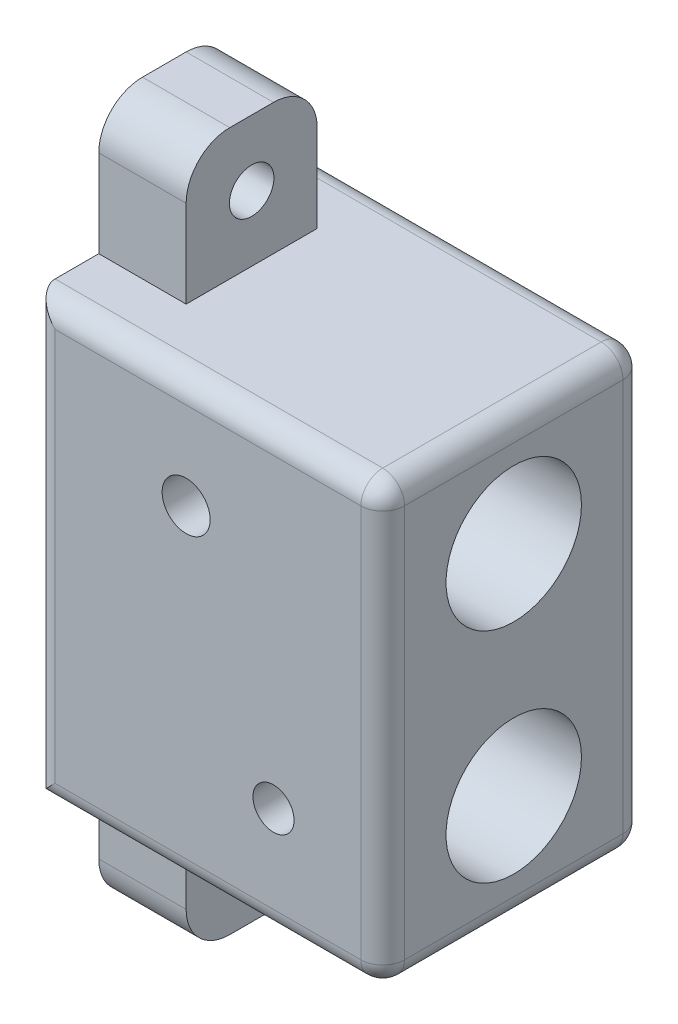
SolidWorks part; units mm, degrees
ref_plane "Front Plane" through (0, 0, 0) normal (0, 0, 1) x (1, 0, 0)
ref_plane "Top Plane" through (0, 0, 0) normal (0, 1, 0) x (1, 0, 0)
ref_plane "Right Plane" through (0, 0, 0) normal (1, 0, 0) x (0, 0, -1)
sketch "Sketch1" plane through (0, 0, 0) normal (0, 1, 0) x (1, 0, 0)
  line L0 (0, 20) -> (20, 20)
  line L2 (0, 0) -> (0, 20)
  line L4 (20, 0) -> (20, 20)
  line L5 (20, 0) -> (80, 0)
  line L6 (0, 0) -> (0, -60)
  line L7 (0, -60) -> (80, -60)
  line L8 (80, 0) -> (80, -60)
  dimension "D1" = 20
  dimension "D2" = 80
  dimension "D3" = 20
  dimension "D4" = 60
extrude "Boss-Extrude1" add sketch "Sketch1" along normal blind 100
sketch "Sketch2" plane through (80, 0, 0) normal (1, 0, 0) x (0, 0, -1)
  line L0 (0, 100) -> (0, 0) construction
  line L1 (0, 100) -> (0, 0) construction
  line L2 (-60, 0) -> (0, 0) construction
  line L3 (-60, 100) -> (0, 100) construction
  circle A0 centre (-30, 75) radius 15.5
  circle A1 centre (-30, 25) radius 15.5
  dimension "D1" = 31
  dimension "D2" = 31
  dimension "D4" = 30
  dimension "D5" = 25
  dimension "D6" = 25
  dimension "D3" = 30
extrude "Cut-Extrude1" cut sketch "Sketch2" against normal blind 70
sketch "Sketch3" plane through (20, 0, 0) normal (1, 0, 0) x (0, 0, -1)
  line L0 (20, 100) -> (20, 0) construction
  line L1 (0, 0) -> (20, 0) construction
  circle A0 centre (10, 87.5) radius 5.1
  circle A1 centre (10, 12.5) radius 5.1
  circle A2 centre (10, 50) radius 5.1
  dimension "D1" = 10
  dimension "D2" = 10
  dimension "D3" = 10.2
  dimension "D4" = 10.2
  dimension "D5" = 75
  dimension "D6" = 12.5
  dimension "D7" = 10
  dimension "D8" = 37.5
  dimension "D9" = 10.2
extrude "Cut-Extrude2" cut sketch "Sketch3" against normal blind 70
sketch "Sketch4" plane through (0, 0, 0) normal (0, 0, -1) x (-1, 0, 0)
  line L0 (-80, 100) -> (-80, 0) construction
  line L1 (-80, 0) -> (-20, 0) construction
  line L2 (-80, 100) -> (-20, 100) construction
  circle A0 centre (-35, 75) radius 5.5
  circle A1 centre (-55, 25) radius 4.7053
  dimension "D1" = 11
  dimension "D2" = 45
  dimension "D3" = 25
  dimension "D4" = 25
  dimension "D5" = 25
extrude "Cut-Extrude3" cut sketch "Sketch4" against normal blind 70
sketch "Sketch5" plane through (0, 0, 0) normal (-1, 0, 0) x (0, 0, 1)
  line L0 (60, 100) -> (60, 0) construction
  line L1 (35, 130) -> (25, 130)
  line L2 (45, 120) -> (45, -20)
  line L3 (35, -30) -> (25, -30)
  line L4 (15, 120) -> (15, -20)
  line L5 (-20, 0) -> (60, 0) construction
  line L6 (-20, 100) -> (60, 100) construction
  circle A0 centre (30, -15) radius 5.1
  circle A1 centre (30, 115) radius 5.1
  arc A2 (25, 130) -> (15, 120) centre (25, 120) ccw
  arc A3 (35, 130) -> (45, 120) centre (35, 120) cw
  arc A4 (45, -20) -> (35, -30) centre (35, -20) cw
  arc A5 (25, -30) -> (15, -20) centre (25, -20) cw
  point P20 (45, -30)
  point P23 (15, -30)
  dimension "D5" = 10.2
  dimension "D6" = 10.2
  dimension "D7" = 15
  dimension "D8" = 15
  dimension "D9" = 15
  dimension "D10" = 15
  dimension "D11" = 10
  dimension "D1" = 30
  dimension "D2" = 15
  dimension "D3" = 30
  dimension "D4" = 30
extrude "Boss-Extrude2" add sketch "Sketch5" against normal blind 20
sketch "Sketch6" plane through (20, 0, 0) normal (1, 0, 0) x (0, 0, -1)
  line L4 (0, 0) -> (20, 0)
  line L5 (20, 0) -> (20, 100)
  line L6 (20, 100) -> (0, 100)
  line L7 (0, 100) -> (0, 0)
  line L8 (0, 0) -> (20, 0)
  line L9 (20, 0) -> (20, 100)
  line L10 (20, 100) -> (0, 100)
  line L11 (0, 100) -> (0, 0)
  dimension "D1" = 0
extrude "Cut-Extrude4" cut sketch "Sketch6" against normal blind 20
fillet "Fillet1" radius 5 10 edges at (0, 50, 60) (40, 100, 60) (40, 0, 60) (80, 0, 30) (80, 50, 60) (80, 100, 30) (0, 50, 0) (80, 50, 0) (40, 0, 0) (40, 100, 0)
